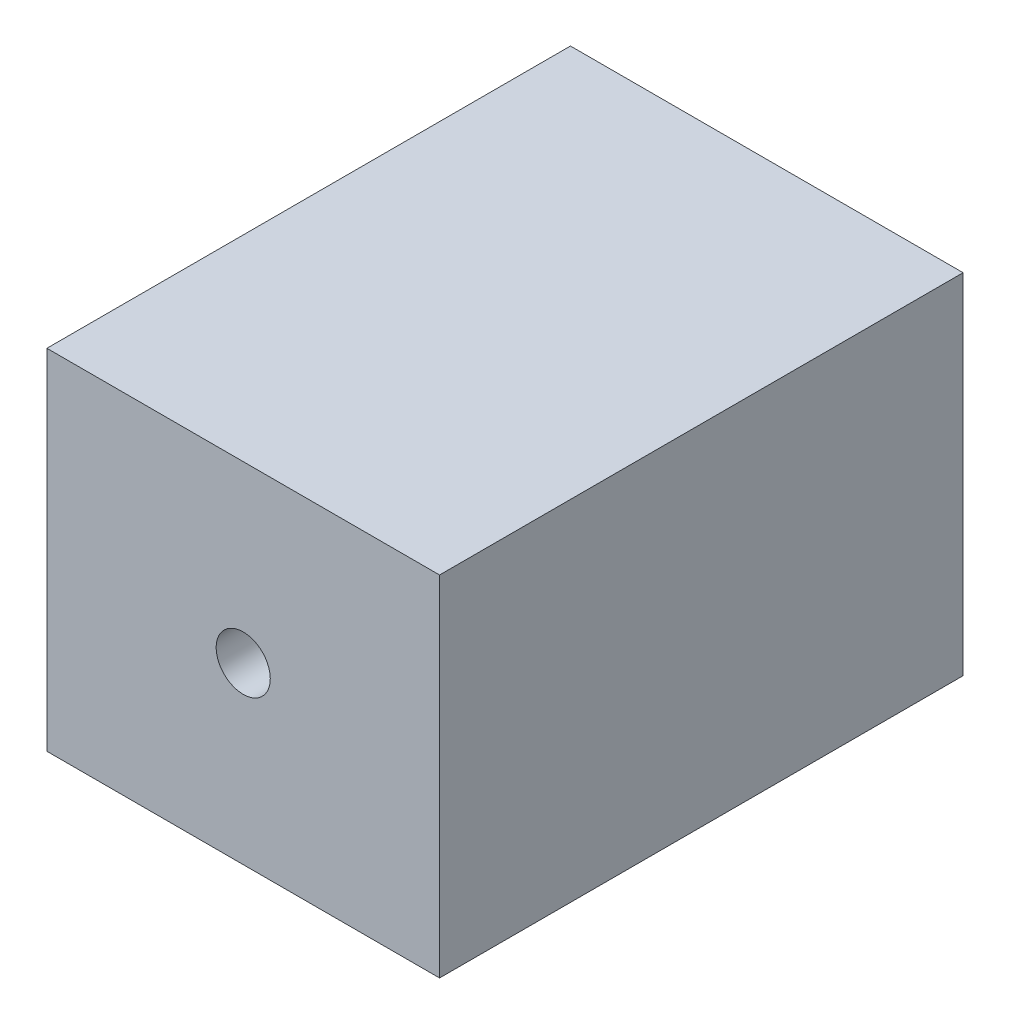
SolidWorks part; units mm, degrees
ref_plane "前视基准面" through (0, 0, 0) normal (0, 0, 1) x (1, 0, 0)
ref_plane "上视基准面" through (0, 0, 0) normal (0, 1, 0) x (1, 0, 0)
ref_plane "右视基准面" through (0, 0, 0) normal (1, 0, 0) x (0, 0, -1)
other "Configuration Table"
sketch "草图1" plane through (0, 0, 0) normal (0, 0, 1) x (1, 0, 0)
  line L0 (-45, -40) -> (45, -40)
  line L1 (45, -40) -> (45, 40)
  line L2 (45, 40) -> (-45, 40)
  line L3 (-45, 40) -> (-45, -40)
  point P0 (0, 0)
  dimension "D1" = 45
  dimension "D2" = 90
  dimension "D3" = 40
  dimension "D4" = 80
extrude "凸台-拉伸1" add sketch "草图1" against normal mid plane 120
sketch "草图2" plane through (0, 0, 0) normal (0, 0, 1) x (1, 0, 0)
  circle A0 centre (0, 0) radius 6.2
  point P0 (0, 0)
  dimension "D1" = 12.4
extrude "切除-拉伸1" cut sketch "草图2" against normal mid plane 160
